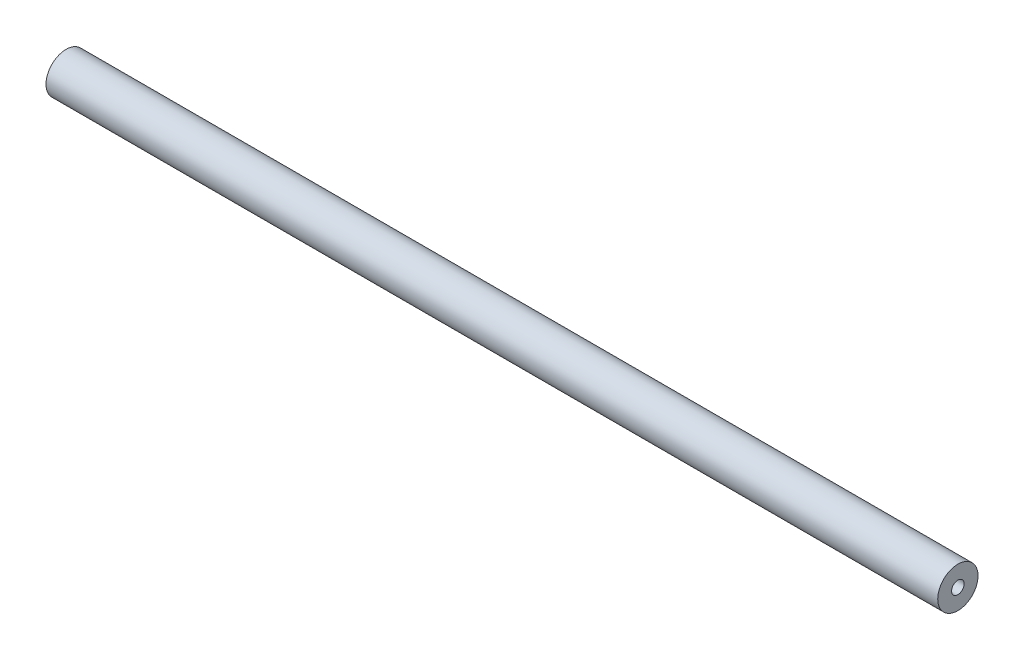
from build123d import *

# Parameters (mm, degrees)
SKETCH1_W             = 354
SKETCH1_H             = 8
M6_TAPPED_HOLE1_D     = 5
M6_TAPPED_HOLE1_DEPTH = 15
M6_TAPPED_HOLE1_TIP   = 1.502151548
M6_TAPPED_HOLE2_D     = 5
M6_TAPPED_HOLE2_DEPTH = 15
M6_TAPPED_HOLE2_TIP   = 1.502151548


with BuildPart() as part:
    # Sketch1 → Revolve1 (revolve)
    with BuildSketch(Plane.XY, mode=Mode.PRIVATE) as revolve1_sk:
        with Locations((0, 4)):
            Rectangle(SKETCH1_W, SKETCH1_H)
    revolve(revolve1_sk.sketch.rotate(Axis((-177, 0, 0), (1, 0, 0)), 90), axis=Axis((-177, 0, 0), (1, 0, 0)))

    # M6 Tapped Hole1
    with Locations(Plane(origin=(177, 0, 0), x_dir=(0, 0, -1), z_dir=(1, 0, 0))):
        with Locations((0, 0)):
            Hole(M6_TAPPED_HOLE1_D / 2, depth=M6_TAPPED_HOLE1_DEPTH)
            with Locations((0, 0, -(M6_TAPPED_HOLE1_DEPTH + M6_TAPPED_HOLE1_TIP / 2))):  # 118° drill point
                Cone(0, M6_TAPPED_HOLE1_D / 2, M6_TAPPED_HOLE1_TIP, mode=Mode.SUBTRACT)

    # M6 Tapped Hole2
    with Locations(Plane.ZY.offset(177)):
        with Locations((0, 0)):
            Hole(M6_TAPPED_HOLE2_D / 2, depth=M6_TAPPED_HOLE2_DEPTH)
            with Locations((0, 0, -(M6_TAPPED_HOLE2_DEPTH + M6_TAPPED_HOLE2_TIP / 2))):  # 118° drill point
                Cone(0, M6_TAPPED_HOLE2_D / 2, M6_TAPPED_HOLE2_TIP, mode=Mode.SUBTRACT)


solid = part.part
